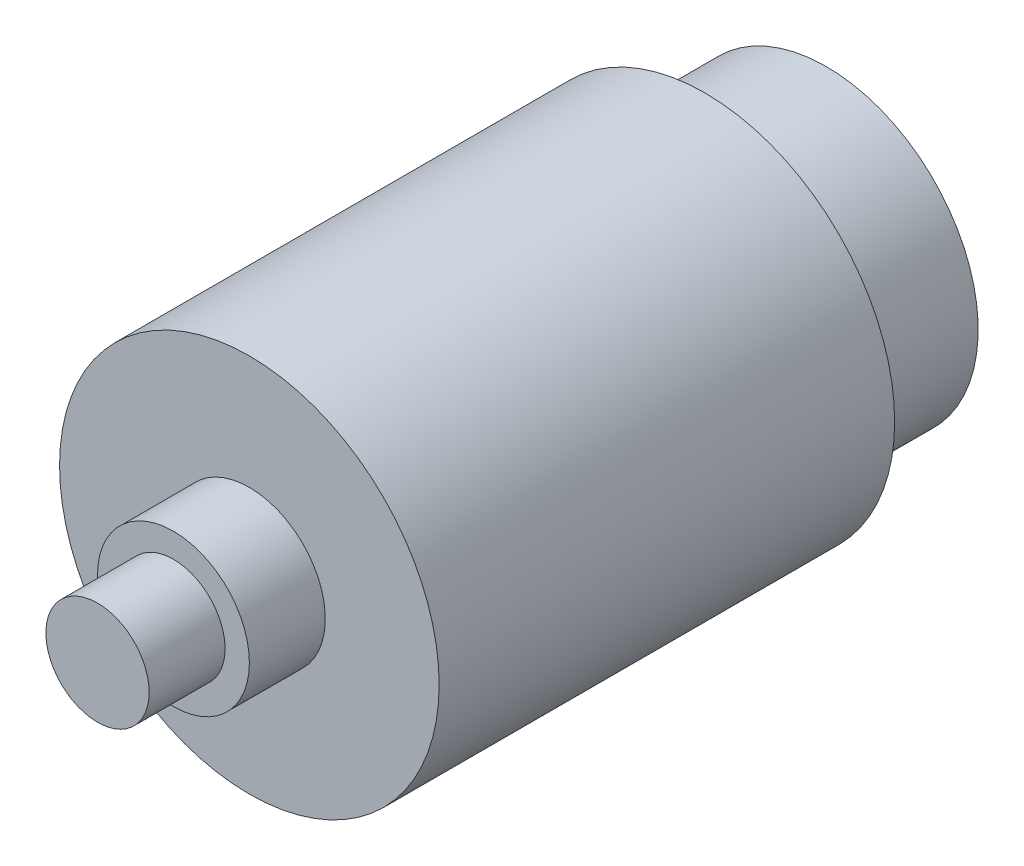
from build123d import *

# Parameters (mm, degrees)
SKETCH1_R           = 5
BOSS_EXTRUDE1_DEPTH = 5
SKETCH2_R           = 3.4
BOSS_EXTRUDE2_DEPTH = 5
SKETCH3_R           = 12.5
BOSS_EXTRUDE3_DEPTH = 30
SKETCH4_R           = 10
BOSS_EXTRUDE4_DEPTH = 8


with BuildPart() as part:
    # Sketch1 → Boss-Extrude1 (new body)
    with BuildSketch(Plane.XY):
        Circle(SKETCH1_R)
    extrude(amount=BOSS_EXTRUDE1_DEPTH)

    # Sketch2 → Boss-Extrude2 (add)
    with BuildSketch(Plane.XY.offset(5)):
        Circle(SKETCH2_R)
    extrude(amount=BOSS_EXTRUDE2_DEPTH)

    # Sketch3 → Boss-Extrude3 (add)
    with BuildSketch(Plane(origin=(0, 0, 0), x_dir=(-1, 0, 0), z_dir=(0, 0, -1))):
        Circle(SKETCH3_R)
    extrude(amount=BOSS_EXTRUDE3_DEPTH)

    # Sketch4 → Boss-Extrude4 (add)
    with BuildSketch(Plane(origin=(0, 0, -30), x_dir=(-1, 0, 0), z_dir=(0, 0, -1))):
        Circle(SKETCH4_R)
    extrude(amount=BOSS_EXTRUDE4_DEPTH)


solid = part.part
